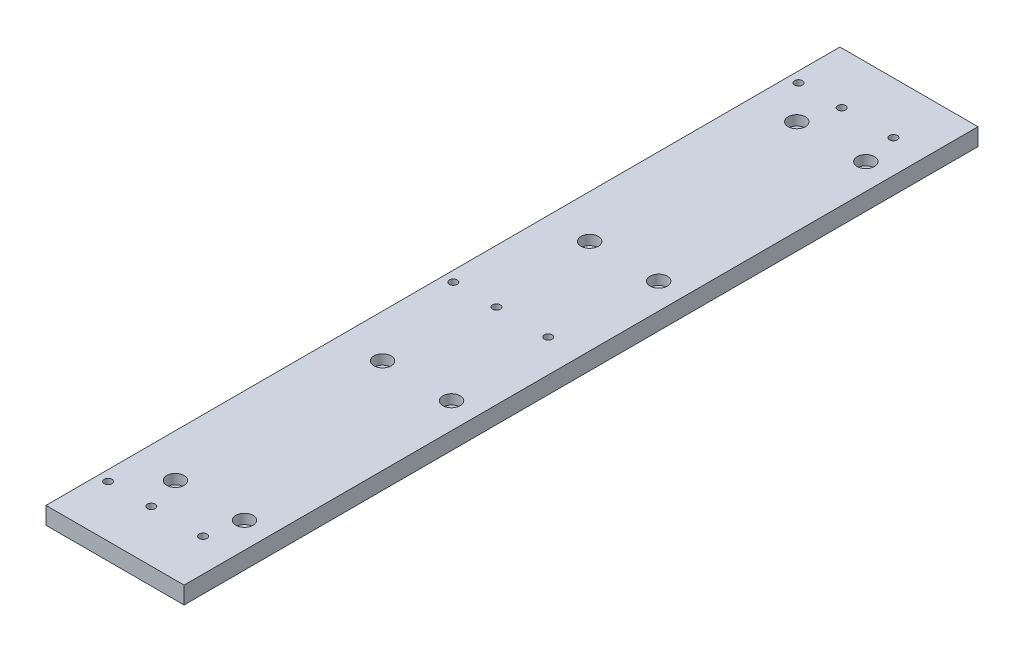
from build123d import *

# Parameters (mm, degrees)
SKETCH_1_W                = 80
SKETCH_1_H                = 10
EXTRUDE_1_DEPTH           = 230
HOLE_WIZARD_1_D           = 4.5
HOLE_WIZARD_1_CBORE_D     = 8
HOLE_WIZARD_1_CBORE_DEPTH = 4.6
HOLE_WIZARD_2_D           = 5.5
HOLE_WIZARD_2_CBORE_D     = 10
HOLE_WIZARD_2_CBORE_DEPTH = 5.7


with BuildPart() as part:
    # 草图1 → 凸台-拉伸1 (new, symmetric)
    with BuildSketch(Plane.XY):
        Rectangle(SKETCH_1_W, SKETCH_1_H)
    extrude(amount=EXTRUDE_1_DEPTH, both=True)

    # 打孔尺寸(%根据)内六角圆柱头螺钉的类型1 (through all)
    with Locations(Plane(origin=(0, -5, 0), x_dir=(-1, 0, 0), z_dir=(0, -1, 0))):
        with Locations((34, -200), (9, -200), (-21, -200), (34, 0), (9, 0), (-21, 0), (34, 200), (9, 200), (-21, 200)):
            CounterBoreHole(HOLE_WIZARD_1_D / 2, HOLE_WIZARD_1_CBORE_D / 2, HOLE_WIZARD_1_CBORE_DEPTH)

    # 打孔尺寸(%根据)内六角圆柱头螺钉的类型2 (through all)
    with Locations(Plane(origin=(0, 5, 0), x_dir=(1, 0, 0), z_dir=(0, 1, 0))):
        with Locations((-15, -180), (25, -180), (-15, -60), (25, -60), (25, 60), (25, 180), (-15, 180), (-15, 60)):
            CounterBoreHole(HOLE_WIZARD_2_D / 2, HOLE_WIZARD_2_CBORE_D / 2, HOLE_WIZARD_2_CBORE_DEPTH)


solid = part.part
